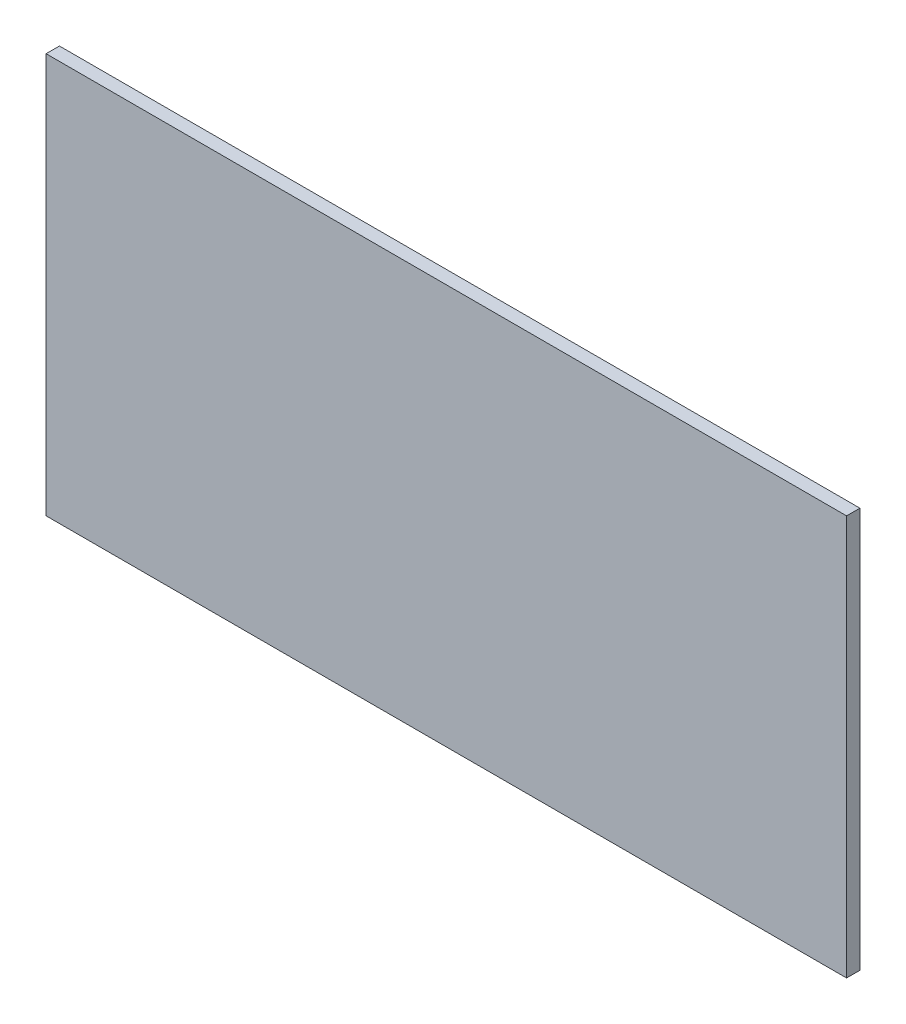
SolidWorks part; units mm, degrees
ref_plane "Front Plane" through (0, 0, 0) normal (0, 0, 1) x (1, 0, 0)
ref_plane "Top Plane" through (0, 0, 0) normal (0, 1, 0) x (1, 0, 0)
ref_plane "Right Plane" through (0, 0, 0) normal (1, 0, 0) x (0, 0, -1)
sketch "Sketch1" plane through (0, 0, 0) normal (0, 0, 1) x (1, 0, 0)
  line L1 (0, 0) -> (300, 0)
  line L2 (0, 0) -> (0, 150)
  line L3 (0, 150) -> (300, 150)
  line L4 (300, 0) -> (300, 150)
  dimension "D1" = 300
  dimension "D2" = 150
extrude "Boss-Extrude1" add sketch "Sketch1" along normal blind 5
